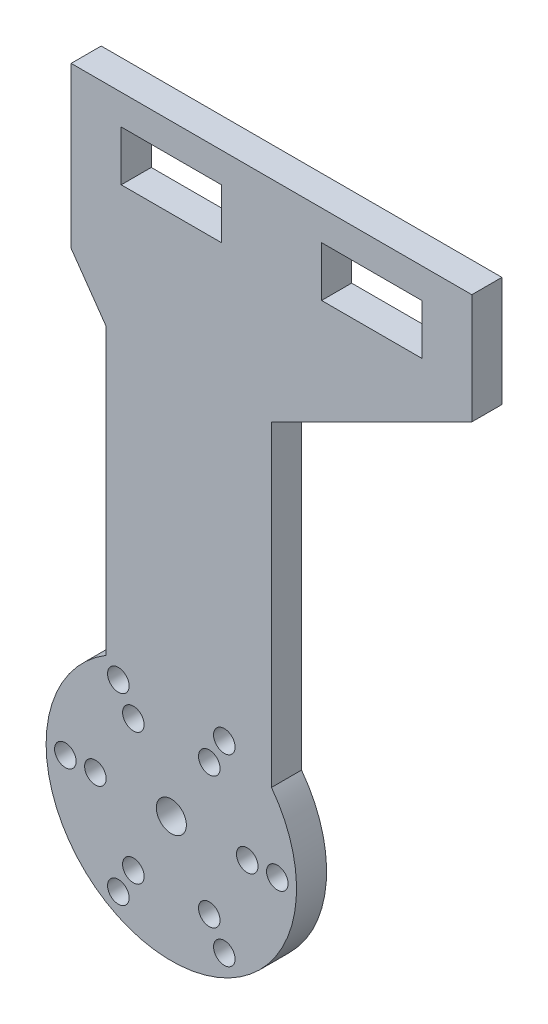
from build123d import *

# Parameters (mm, degrees)
SKETCH_1_R      = 1.5
SKETCH_1_R_2    = 1.075
SKETCH_1_W      = 10
SKETCH_1_H      = 5
EXTRUDE_1_DEPTH = 3


with BuildPart() as part:
    # 草图1 → 凸台-拉伸1 (new body)
    with BuildSketch(Plane.XY):
        with BuildLine():
            Line((-15.405029449, -13.33425996), (-15.405029449, 15.090143764))
            Line((-15.405029449, 15.090143764), (-18.905029449, 20.088661788))
            Line((-18.905029449, 20.088661788), (-18.905029449, 36.088661788))
            Line((-18.905029449, 36.088661788), (21.094970551, 36.088661788))
            Line((21.094970551, 36.088661788), (21.094970551, 25.088661788))
            Line((21.094970551, 25.088661788), (1.094970551, 15.088661788))
            Line((1.094970551, 15.088661788), (1.094970551, -16.511338212))
            ThreePointArc((1.094970551, -16.511338212), (-11.26849228, -36.285866449), (-15.405029449, -13.33425996))
        make_face()
        with Locations((-8.905029449, -24.011338212)):
            Circle(SKETCH_1_R, mode=Mode.SUBTRACT)
        with Locations((-1.325029449, -24.011338212)):
            Circle(SKETCH_1_R_2, mode=Mode.SUBTRACT)
        with Locations((1.674970551, -24.011338212)):
            Circle(SKETCH_1_R_2, mode=Mode.SUBTRACT)
        with Locations((-5.115029449, -30.575810773)):
            Circle(SKETCH_1_R_2, mode=Mode.SUBTRACT)
        with Locations((-3.615029449, -33.173886984)):
            Circle(SKETCH_1_R_2, mode=Mode.SUBTRACT)
        with Locations((-12.695029449, -30.575810773)):
            Circle(SKETCH_1_R_2, mode=Mode.SUBTRACT)
        with Locations((-14.195029449, -33.173886984)):
            Circle(SKETCH_1_R_2, mode=Mode.SUBTRACT)
        with Locations((-16.485029449, -24.011338212)):
            Circle(SKETCH_1_R_2, mode=Mode.SUBTRACT)
        with Locations((-19.485029449, -24.011338212)):
            Circle(SKETCH_1_R_2, mode=Mode.SUBTRACT)
        with Locations((-12.695029449, -17.446865652)):
            Circle(SKETCH_1_R_2, mode=Mode.SUBTRACT)
        with Locations((-14.195029449, -14.84878944)):
            Circle(SKETCH_1_R_2, mode=Mode.SUBTRACT)
        with Locations((-5.115029449, -17.446865652)):
            Circle(SKETCH_1_R_2, mode=Mode.SUBTRACT)
        with Locations((-3.615029449, -14.84878944)):
            Circle(SKETCH_1_R_2, mode=Mode.SUBTRACT)
        with Locations((-8.905029449, 30.588661788)):
            Rectangle(SKETCH_1_W, SKETCH_1_H, mode=Mode.SUBTRACT)
        with Locations((11.094970551, 30.588661788)):
            Rectangle(SKETCH_1_W, SKETCH_1_H, mode=Mode.SUBTRACT)
    extrude(amount=EXTRUDE_1_DEPTH)


solid = part.part
